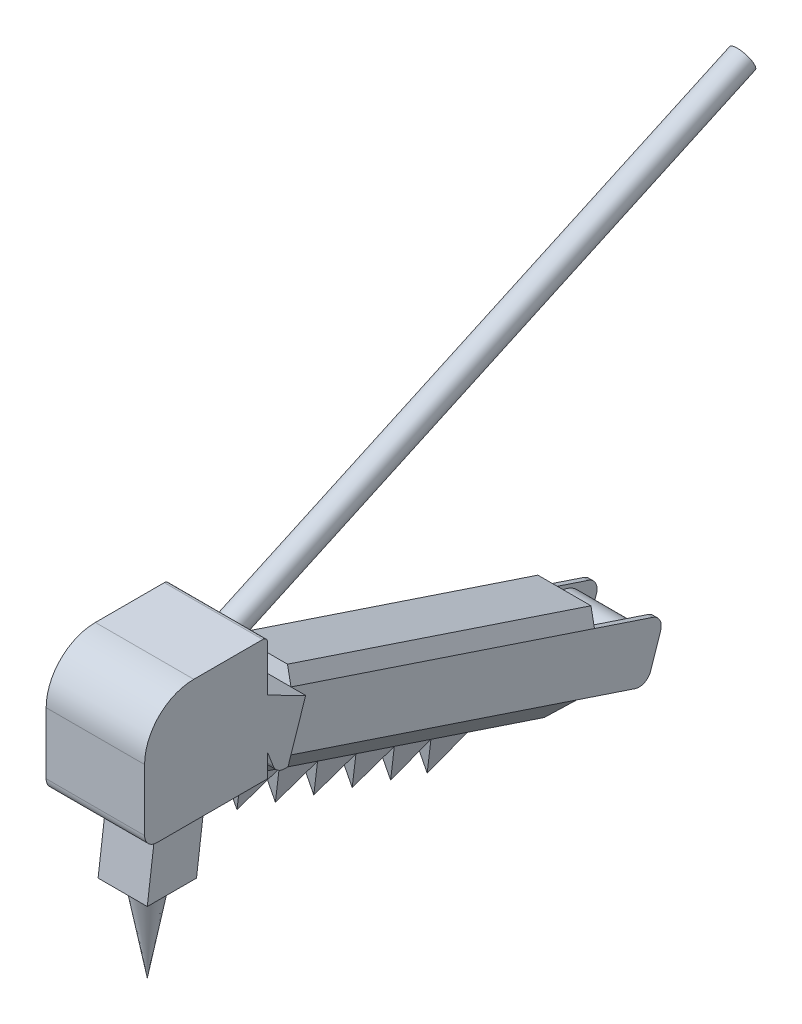
from build123d import *

# Parameters (mm, degrees)
BOSS_EXTRUDE1_DEPTH  = 40
FILLET1_R            = 20
FILLET2_R            = 5
BOSS_EXTRUDE2_DEPTH  = 10
FILLET3_R            = 5
FILLET4_R            = 2
BOSS_EXTRUDE6_DEPTH  = 100
BOSS_EXTRUDE8_DEPTH  = 4
CUT_EXTRUDE5_DEPTH   = 102
BOSS_EXTRUDE14_DEPTH = 30
CUT_EXTRUDE4_DEPTH   = 100
SKETCH25_W           = 2
SKETCH25_H           = 22.692372085
SKETCH25_H_2         = 22.697350811
BOSS_EXTRUDE15_DEPTH = 30
SKETCH26_R           = 10
BOSS_EXTRUDE16_DEPTH = 26.073999752
FILLET5_R            = 5


with BuildPart() as part:
    # Sketch2 → Boss-Extrude1 (new body)
    with BuildSketch(Plane(origin=(0, 0, 0), x_dir=(0, 0, -1), z_dir=(1, 0, 0))):
        Polygon((0, 0), (0, 50), (50, 50), (50, 29.410176709), (65.452441178, 21.589257338), (58.276483048, 0.061382948), (53.5278156, 0.061382948), (50, 9.231987855), (50, 0), align=None)
    extrude(amount=BOSS_EXTRUDE1_DEPTH)

    # Fillet1
    fillet1_edges = [part.edges().sort_by_distance(p)[0] for p in [
        (20, 50, 0),
    ]]
    fillet(fillet1_edges, radius=FILLET1_R)

    # Fillet2
    fillet2_edges = [part.edges().sort_by_distance(p)[0] for p in [
        (20, 0, 0),
    ]]
    fillet(fillet2_edges, radius=FILLET2_R)

    # Sketch4 → Boss-Extrude2 (add, symmetric)
    with BuildSketch(Plane(origin=(20, 0, 0), x_dir=(0, 0, -1), z_dir=(1, 0, 0))):
        Polygon((15, 0), (11.097402588, -30.529005874), (31.097402588, -30.529005874), (35, 0), align=None)
    extrude(amount=BOSS_EXTRUDE2_DEPTH, both=True)

    # Sketch5 → Revolve1 (revolve)
    with BuildSketch(Plane(origin=(20, 0, 0), x_dir=(0, 0, -1), z_dir=(1, 0, 0)), mode=Mode.PRIVATE) as revolve1_sk:
        Polygon((21.097402588, -30.529005874), (27.664898482, -30.529005874), (21.097402588, -65.678202337), align=None)
    revolve(revolve1_sk.sketch.rotate(Axis((20, -30.529005874, -21.097402588), (0, -1, 0)), 180), axis=Axis((20, -30.529005874, -21.097402588), (0, -1, 0)))

    # Fillet3
    fillet3_edges = [part.edges().sort_by_distance(p)[0] for p in [
        (20, 0.061382948, -53.5278156),
    ]]
    fillet(fillet3_edges, radius=FILLET3_R)

    # Fillet4
    fillet4_edges = [part.edges().sort_by_distance(p)[0] for p in [
        (20, 50, -50),
    ]]
    fillet(fillet4_edges, radius=FILLET4_R)

    # Sketch7 → Boss-Extrude6 (add)
    with BuildSketch(Plane(origin=(0, -17.47680662, -52.430419859), x_dir=(-1, 0, 0), z_dir=(0, -0.3162277660168374, -0.9486832980505141))):
        Polygon((-5.963000124, 18.486875023), (-16, 8.348197136), (-24, 8.348197136), (-34.036999876, 18.486875023), (-34.036999876, 46.955249244), (-5.963000124, 46.955249244), align=None)
    extrude(amount=BOSS_EXTRUDE6_DEPTH)

    # Sketch10 → Boss-Extrude8 (add, symmetric)
    with BuildSketch(Plane(origin=(20, 0, 0), x_dir=(0, 0, -1), z_dir=(1, 0, 0))):
        Polygon((147.227393234, -40.276025309), (132.358652474, -35.319778389), (134.836775442, -50.433902239), align=None)
        Polygon((132.358652474, -35.319778389), (117.489911715, -30.363531469), (119.968034683, -45.477655319), align=None)
        Polygon((117.489911715, -30.363531469), (101.885021683, -25.161901459), (104.363144652, -40.276025309), align=None)
        Polygon((101.885021683, -25.161901459), (86.280131652, -19.960271448), (88.75825462, -35.074395299), align=None)
        Polygon((86.280131652, -19.960271448), (70.675241621, -14.758641438), (73.153364589, -29.872765288), align=None)
        Polygon((70.675241621, -14.758641438), (55.07035159, -9.557011428), (57.548474558, -24.671135278), align=None)
    extrude(amount=BOSS_EXTRUDE8_DEPTH, both=True)

    # Sketch23 → Cut-Extrude5 (cut)
    with BuildSketch(Plane(origin=(0, -49.099583221, -147.298749664), x_dir=(-1, 0, 0), z_dir=(0, -0.3162277660168373, -0.948683298050514))):
        Polygon((-16, -5.206668435), (-16, 8.348197136), (-20, -5.214113496), align=None)
        Polygon((-24, -5.206668435), (-24, 8.348197136), (-20, -5.214113496), align=None)
    extrude(amount=-CUT_EXTRUDE5_DEPTH, mode=Mode.SUBTRACT)

    # Sketch24 → Boss-Extrude14 (add)
    with BuildSketch(Plane(origin=(0, -49.099583221, -147.298749664), x_dir=(-1, 0, 0), z_dir=(0, -0.3162277660168373, -0.948683298050514))):
        Polygon((-5.963000124, 18.486875023), (-5.963000124, 46.955249244), (-34.036999876, 46.955249244), (-34.036999876, 18.486875023), (-24, 8.348197136), (-16, 8.348197136), align=None)
    extrude(amount=BOSS_EXTRUDE14_DEPTH)

    # Sketch20 → Cut-Extrude4 (cut, symmetric)
    with BuildSketch(Plane(origin=(0, -49.099583221, -147.298749664), x_dir=(-1, 0, 0), z_dir=(0, -0.3162277660168373, -0.948683298050514))):
        Polygon((-34.036999876, 41.184225834), (-30.780503979, 46.955249244), (-34.036999876, 46.955249244), align=None)
        Polygon((-5.963000124, 41.184225834), (-9.219496021, 46.955249244), (-5.963000124, 46.955249244), align=None)
    extrude(amount=CUT_EXTRUDE4_DEPTH, both=True, mode=Mode.SUBTRACT)

    # Sketch25 → Boss-Extrude15 (add)
    with BuildSketch(Plane(origin=(0, -58.586416202, -175.759248606), x_dir=(-1, 0, 0), z_dir=(0, -0.31622776601683655, -0.9486832980505142))):
        with Locations((-33.036999876, 29.833061066)):
            Rectangle(SKETCH25_W, SKETCH25_H)
        with Locations((-6.963000124, 29.835550428)):
            Rectangle(SKETCH25_W, SKETCH25_H_2)
    extrude(amount=BOSS_EXTRUDE15_DEPTH)

    # Sketch26 → Boss-Extrude16 (add)
    with BuildSketch(Plane(origin=(34.036999876, 0, 0), x_dir=(0, 0, -1), z_dir=(1, 0, 0))):
        with Locations((200.721074436, -35.457593279)):
            Circle(SKETCH26_R)
    extrude(amount=-BOSS_EXTRUDE16_DEPTH)

    # Fillet5
    fillet5_edges = [part.edges().sort_by_distance(p)[0] for p in [
        (33.036999876, -50.535059615, -210.065810737),
        (33.036999876, -29.007185225, -217.241768866),
        (6.963000124, -29.00246199, -217.243343278),
        (6.963000124, -50.535059615, -210.065810737),
    ]]
    fillet(fillet5_edges, radius=FILLET5_R)

    # Sketch28 → Revolve3 (revolve)
    with BuildSketch(Plane(origin=(20, 0, 0), x_dir=(0, 0, -1), z_dir=(1, 0, 0))):
        Polygon((50, 33.769630528), (50, 39.271662622), (262.981733141, 137.079749362), (265.068381635, 132.535973612), align=None)
    revolve(axis=Axis((20, 39.271662622, -50), (0, 0.4173296987488473, -0.9087551499398484)))


solid = part.part
